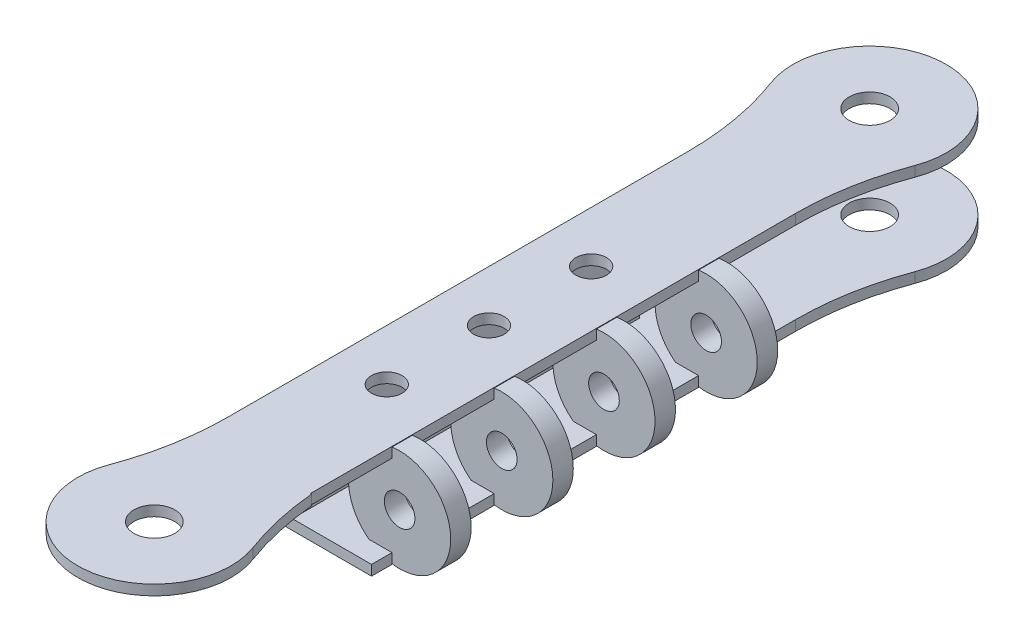
SolidWorks part; units mm, degrees
ref_plane "Front Plane" through (0, 0, 0) normal (0, 0, 1) x (1, 0, 0)
ref_plane "Top Plane" through (0, 0, 0) normal (0, 1, 0) x (1, 0, 0)
ref_plane "Right Plane" through (0, 0, 0) normal (1, 0, 0) x (0, 0, -1)
other "Configuration Table"
sketch "Sketch1" plane through (0, 0, 0) normal (0, 1, 0) x (1, 0, 0)
  line L0 (0, -35) -> (-76.7842, -35) construction
  line L1 (-5.2547, -12.5) -> (-5.2547, -57.5)
  line L3 (0, 0) -> (0, -70) construction
  line L4 (5.2547, -12.5) -> (5.2547, -57.5)
  arc A0 (7.5, 0) -> (-7.5, 0) centre (0, 0) ccw
  arc A1 (-7.5, -70) -> (7.5, -70) centre (0, -70) ccw
  arc A2 (-7.5, 0) -> (-7.0312, -2.6101) centre (0, 0) ccw
  arc A3 (-7.0312, -2.6101) -> (-5.2547, -12.5) centre (-33.6728, -12.5) cw
  arc A4 (-7.0312, -67.3899) -> (-5.2547, -57.5) centre (-33.6728, -57.5) ccw
  arc A5 (-7.5, -70) -> (-7.0312, -67.3899) centre (0, -70) cw
  arc A6 (7.0312, -67.3899) -> (5.2547, -57.5) centre (33.6728, -57.5) cw
  arc A7 (7.0312, -2.6101) -> (5.2547, -12.5) centre (33.6728, -12.5) ccw
  arc A8 (7.5, -70) -> (7.0312, -67.3899) centre (0, -70) ccw
  arc A9 (7.0312, -2.6101) -> (7.5, 0) centre (0, 0) ccw
  dimension "D1" = 15
  dimension "D3" = 45
  dimension "D2" = 70
extrude "Boss-Extrude1" add sketch "Sketch1" along normal blind 10
sketch "Sketch2" plane through (0, 10, 0) normal (0, 1, 0) x (1, 0, 0)
  circle A0 centre (0, 0) radius 2
  circle A1 centre (0, -70) radius 2
  dimension "D1" = 4
  dimension "D2" = 4
extrude "Cut-Extrude1" cut sketch "Sketch2" against normal through all both and the other way through all
sketch "Sketch5" plane through (0, 0, 0) normal (0, 0, 1) x (1, 0, 0)
  line L0 (7.5, 9) -> (-2.5, 9)
  line L1 (7.5, 0) -> (7.5, 10) construction
  line L2 (-2.5, 9) -> (-2.5, 1)
  line L3 (-2.5, 1) -> (7.5, 1)
  line L4 (7.5, 1) -> (7.5, 9)
  line L5 (7.5, 10) -> (-7.5, 10) construction
  line L6 (-7.5, 0) -> (7.5, 0) construction
  line L7 (-7.5, 10) -> (-7.5, 0) construction
  dimension "D1" = 1
  dimension "D2" = 1
  dimension "D3" = 5
extrude "Cut-Extrude4" cut sketch "Sketch5" against normal through all both and the other way through all
ref_plane "Plane1" through (0, 0, 20) normal (0, 0, 1) x (1, 0, 0)
sketch "Sketch3" plane through (0, 0, 20) normal (0, 0, 1) x (1, 0, 0)
  line L0 (-7.5, 0) -> (7.5, 0) construction
  circle A0 centre (6, 5) radius 5
  dimension "D1" = 6
  dimension "D2" = 10
  dimension "D3" = 5
extrude "Boss-Extrude2" add sketch "Sketch3" along normal blind 40
sketch "Sketch4" plane through (0, 0, 0) normal (0, 1, 0) x (1, 0, 0)
  line L0 (9.2547, -22) -> (5.2547, -22)
  line L1 (5.2547, -12.5) -> (5.2547, -60) construction
  line L2 (5.2547, -22) -> (5.2547, -30)
  line L3 (5.2547, -30) -> (9.2547, -30)
  line L4 (9.2547, -30) -> (9.2547, -22)
  line L5 (5.2547, -32) -> (5.2547, -40)
  line L6 (9.2547, -40) -> (9.2547, -32)
  line L7 (-5.5, -20) -> (5.5, -20) construction
  line L8 (5.2547, -40) -> (9.2547, -40)
  line L9 (9.2547, -32) -> (5.2547, -32)
  line L10 (5.2547, -42) -> (5.2547, -50)
  line L11 (9.2547, -50) -> (9.2547, -42)
  line L12 (5.2547, -50) -> (9.2547, -50)
  line L13 (9.2547, -42) -> (5.2547, -42)
  line L14 (5.2547, -32) -> (5.2547, -40)
  line L15 (9.2547, -40) -> (9.2547, -32)
  line L16 (5.2547, -40) -> (9.2547, -40)
  line L17 (9.2547, -32) -> (5.2547, -32)
  line L18 (9.2547, -60) -> (9.2547, -52)
  line L19 (9.2547, -52) -> (5.2547, -52)
  line L20 (5.2547, -52) -> (5.2547, -60)
  line L21 (5.2547, -60) -> (9.2547, -60)
  dimension "D1" = 8
  dimension "D2" = 10
  dimension "D3" = 4
  dimension "D4" = 2
  dimension "D5" = 2
  dimension "D6" = 2
extrude "Cut-Extrude3" cut sketch "Sketch4" against normal through all both and the other way through all contours L6 L9 L5 L8 | L4 L0 L2 L3 | L11 L13 L10 L12 | L18 L19 L20 L21
sketch "Sketch6" plane through (5.2547, 0, 0) normal (1, 0, 0) x (0, 0, -1)
  line L0 (-60, 8.9992) -> (-50, 9) construction
  line L1 (-20, 9) -> (-12.5, 9) construction
  line L2 (-60, 1) -> (-20, 1) construction
  line L3 (-20, 5.5) -> (-20, -5.5) construction
  line L4 (7.0711, 1) -> (-77.0711, 1) construction
  line L6 (-60, 8.9992) -> (-52, 8.9992)
  line L7 (-60, 8.9992) -> (-60, 1)
  line L8 (-60, 1) -> (-52, 1)
  line L9 (-52, 8.9992) -> (-52, 1)
  line L10 (-52, 10) -> (-52, 8.7956) construction
  line L11 (-50, 0.0559) -> (-50, 9.9441) construction
  line L12 (-50, 9) -> (-42, 9)
  line L13 (-50, 9) -> (-50, 1)
  line L14 (-50, 1) -> (-42, 1)
  line L15 (-42, 9) -> (-42, 1)
  line L16 (-40, 0) -> (-40, 1.2044) construction
  line L17 (-40, 9.0008) -> (-32, 9.0008)
  line L18 (-40, 9.0008) -> (-40, 1)
  line L19 (-40, 1) -> (-32, 1)
  line L20 (-32, 9.0008) -> (-32, 1)
  line L21 (-30, 0.0559) -> (-30, 9.9441) construction
  line L22 (-30, 9.0016) -> (-22, 9.0016)
  line L23 (-30, 9.0016) -> (-30, 1)
  line L24 (-30, 1) -> (-22, 1)
  line L25 (-22, 9.0016) -> (-22, 1)
  line L26 (-22, 0.0559) -> (-22, 9.9441) construction
  dimension "D1" = 8
  dimension "D2" = 8
  dimension "D3" = 7.9992
  dimension "D4" = 8
extrude "Cut-Extrude5" cut sketch "Sketch6" against normal blind 5 and the other way through all
sketch "Sketch7" plane through (0, 0, 20) normal (0, 0, 1) x (1, 0, 0)
  line L0 (-2.5, 9) -> (-7.5, 9)
  line L1 (-7.5, 10) -> (-7.5, 0) construction
  line L2 (-2.5, 9) -> (-2.5, 1)
  line L3 (-2.5, 1) -> (-7.5, 1)
  line L4 (-7.5, 1) -> (-7.5, 9)
extrude "Cut-Extrude6" cut sketch "Sketch7" against normal through all
sketch "Sketch9" plane through (0, 10, 0) normal (0, 1, 0) x (1, 0, 0)
  line L0 (-0.2547, -20) -> (-0.2547, -49.9755) construction
  line L1 (-5.5, -20) -> (5.5, -20) construction
  line L2 (-0.2547, -49.9755) -> (5.2547, -49.9755) construction
  line L3 (5.2547, -60) -> (5.2547, -12.5) construction
  line L4 (5.2547, -49.9755) -> (5.2547, -20) construction
  line L5 (5.2547, -20) -> (-0.2547, -20) construction
  line L6 (-5.2547, -12.5) -> (-5.2547, -57.5) construction
  circle A0 centre (-0.2547, -27) radius 1.5
  circle A1 centre (-0.2547, -37) radius 1.5
  circle A2 centre (-0.2547, -47) radius 1.5
  dimension "D1" = 3
  dimension "D2" = 3
  dimension "D3" = 3
  dimension "D4" = 7
  dimension "D5" = 17
  dimension "D6" = 27
  dimension "D7" = 5
extrude "Cut-Extrude8" cut sketch "Sketch9" against normal through all both and the other way through all
sketch "Sketch10" plane through (0, 0, 52) normal (0, 0, 1) x (1, 0, 0)
  circle A0 centre (6, 5) radius 1.5
  dimension "D1" = 3
extrude "Cut-Extrude9" cut sketch "Sketch10" against normal through all both and the other way through all
ref_plane "Plane2" through (0, 0, 60) normal (0, 0, 1) x (1, 0, 0)
sketch "Sketch11" plane through (0, 0, 60) normal (0, 0, 1) x (1, 0, 0)
  line L0 (8.6645, 9) -> (-9.3355, 9)
  line L1 (-2.5, 9) -> (7.5, 9) construction
  line L2 (-9.3355, 9) -> (-9.3355, 0)
  line L3 (-9.3355, 0) -> (8.6645, 0)
  line L4 (8.6645, 9) -> (8.6645, 0)
  dimension "D1" = 18
extrude "Cut-Extrude10" cut sketch "Sketch11" along normal through all
sketch "Sketch12" plane through (0, 0, 60) normal (0, 0, 1) x (1, 0, 0)
  line L6 (5.2547, 0) -> (5.2547, 1)
  line L7 (5.2547, 1) -> (-2.5, 1)
  line L8 (-2.5, 1) -> (-2.5, 9)
  line L9 (-2.5, 9) -> (-5.3649, 9)
  line L10 (-5.3649, 9) -> (-5.3649, 0)
  line L11 (-5.3649, 0) -> (5.2547, 0)
  line L12 (5.2547, 0) -> (5.2547, 1)
  line L13 (5.2547, 1) -> (-2.5, 1)
  line L14 (-2.5, 1) -> (-2.5, 9)
  line L15 (-2.5, 9) -> (-5.3649, 9)
  line L16 (-5.3649, 9) -> (-5.3649, 0)
  line L17 (-5.3649, 0) -> (5.2547, 0)
  dimension "D1" = 0
extrude "Cut-Extrude11" cut sketch "Sketch12" against normal blind 6
